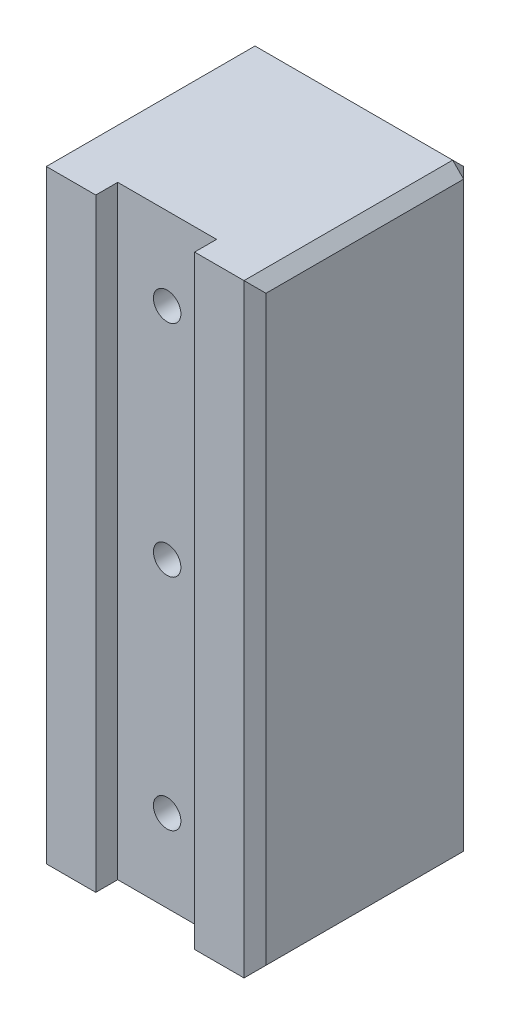
SolidWorks part; units mm, degrees
material "A6061"
ref_plane "Front Plane" through (0, 0, 0) normal (0, 0, 1) x (1, 0, 0)
ref_plane "Top Plane" through (0, 0, 0) normal (0, 1, 0) x (1, 0, 0)
ref_plane "Right Plane" through (0, 0, 0) normal (1, 0, 0) x (0, 0, -1)
sketch "Sketch1" plane through (0, 0, 0) normal (0, 0, 1) x (1, 0, 0)
  line L1 (-10, -27.5) -> (10, -27.5)
  line L2 (-10, -27.5) -> (-10, 27.5)
  line L3 (-10, 27.5) -> (10, 27.5)
  line L4 (10, -27.5) -> (10, 27.5)
  line L5 (-10, -27.5) -> (10, 27.5) construction
  line L6 (-10, 27.5) -> (10, -27.5) construction
  point P0 (0, 0)
  dimension "D1" = 20
  dimension "D2" = 55
extrude "Boss-Extrude1" add sketch "Sketch1" along normal blind 20
sketch "Sketch2" plane through (0, 0, 20) normal (0, 0, 1) x (1, 0, 0)
  line L0 (10, 27.5) -> (-10, 27.5) construction
  line L1 (-4.5, -27.5) -> (4.5, -27.5)
  line L2 (-4.5, -27.5) -> (-4.5, 27.5)
  line L3 (-4.5, 27.5) -> (4.5, 27.5)
  line L4 (4.5, -27.5) -> (4.5, 27.5)
  line L5 (-4.5, -27.5) -> (4.5, 27.5) construction
  line L6 (-4.5, 27.5) -> (4.5, -27.5) construction
  point P0 (0, 0)
  dimension "D1" = 9
extrude "Cut-Extrude1" cut sketch "Sketch2" against normal blind 2
hole_wizard "M3 Tapped Hole1" positions "Sketch4" profile "Sketch3" tap size "M3" standard "GB"
sketch "Sketch4" plane through (0, 0, 18) normal (0, 0, 1) x (1, 0, 0)
  line L0 (0, -27.5) -> (0, 27.5)
  line L1 (-4.5, -27.5) -> (4.5, -27.5) construction
  line L2 (4.5, 27.5) -> (-4.5, 27.5) construction
  line L4 (10, 27.5) -> (4.5, 27.5) construction
  point P0 (0, 20)
  point P2 (0, 0)
  point P4 (0, -20)
  dimension "D1" = 7.5
  dimension "D2" = 20
  dimension "D3" = 20
cosmetic thread "Cosmetic Thread1" parameters "D1"=6, "D2"=3
cosmetic thread "Cosmetic Thread2" parameters "D1"=6, "D2"=3
cosmetic thread "Cosmetic Thread3" parameters "D1"=6, "D2"=3
sketch "Sketch3" plane through (0, 20, 18) normal (1, 0, 0) x (0, -1, 0)
  line L0 (0, 0) -> (0, 8.2511)
  line L1 (0, 8.2511) -> (1.25, 7.5)
  line L2 (1.25, 7.5) -> (1.25, 0)
  line L5 (1.25, 0) -> (0, 0)
  line L10 (0, 8.2511) -> (-1.25, 7.5) construction
  line L11 (0, -6.35) -> (0, 107.95) construction
  dimension "螺纹孔钻头直径" = 2.5
  dimension "螺纹孔钻头深度" = 7.5
  dimension "导头角度" = 118
hole_wizard "M4 Tapped Hole1" positions "Sketch6" profile "Sketch5" tap size "M4" standard "GB"
sketch "Sketch6" plane through (0, -27.5, 0) normal (0, -1, 0) x (-1, 0, 0)
  line L1 (4.5, -18) -> (-4.5, -18) construction
  point P0 (0, -13)
  point P2 (0, -5.5)
  dimension "D1" = 5
  dimension "D2" = 7.5
sketch "Sketch5" plane through (0, -27.5, 13) normal (1, 0, 0) x (0, 0, -1)
  line L0 (0, 0) -> (0, 11.0914)
  line L1 (0, 11.0914) -> (1.65, 10.1)
  line L2 (1.65, 10.1) -> (1.65, 0)
  line L5 (1.65, 0) -> (0, 0)
  line L10 (0, 11.0914) -> (-1.65, 10.1) construction
  line L11 (0, -6.35) -> (0, 107.95) construction
  dimension "螺纹孔钻头直径" = 3.3
  dimension "螺纹孔钻头深度" = 10.1
  dimension "导头角度" = 118
cosmetic thread "Cosmetic Thread4" parameters "D1"=8, "D2"=4
cosmetic thread "Cosmetic Thread5" parameters "D1"=8, "D2"=4
hole_wizard "M5 Tapped Hole1" positions "Sketch8" profile "Sketch7" tap size "M5" standard "GB"
sketch "Sketch8" plane through (0, 0, 0) normal (0, 0, -1) x (-1, 0, 0)
  point P0 (0, 20)
  point P3 (0, -20)
sketch "Sketch7" plane through (0, 20, 0) normal (1, 0, 0) x (0, 1, 0)
  line L0 (0, 0) -> (0, 13.6618)
  line L1 (0, 13.6618) -> (2.1, 12.4)
  line L2 (2.1, 12.4) -> (2.1, 0)
  line L5 (2.1, 0) -> (0, 0)
  line L10 (0, 13.6618) -> (-2.1, 12.4) construction
  line L11 (0, -6.35) -> (0, 107.95) construction
  dimension "螺纹孔钻头直径" = 4.2
  dimension "螺纹孔钻头深度" = 12.4
  dimension "导头角度" = 118
cosmetic thread "Cosmetic Thread6" parameters "D1"=10, "D2"=5
cosmetic thread "Cosmetic Thread7" parameters "D1"=10, "D2"=5
chamfer "Chamfer1" distance 1 angle 45 10 edges at (-10, -27.5, 10) (10, -27.5, 10) (0, -27.5, 0) (10, 0, 0) (10, 0, 20) (-10, 0, 20) (-10, 0, 0) (-10, 27.5, 10) (0, 27.5, 0) (10, 27.5, 10)
